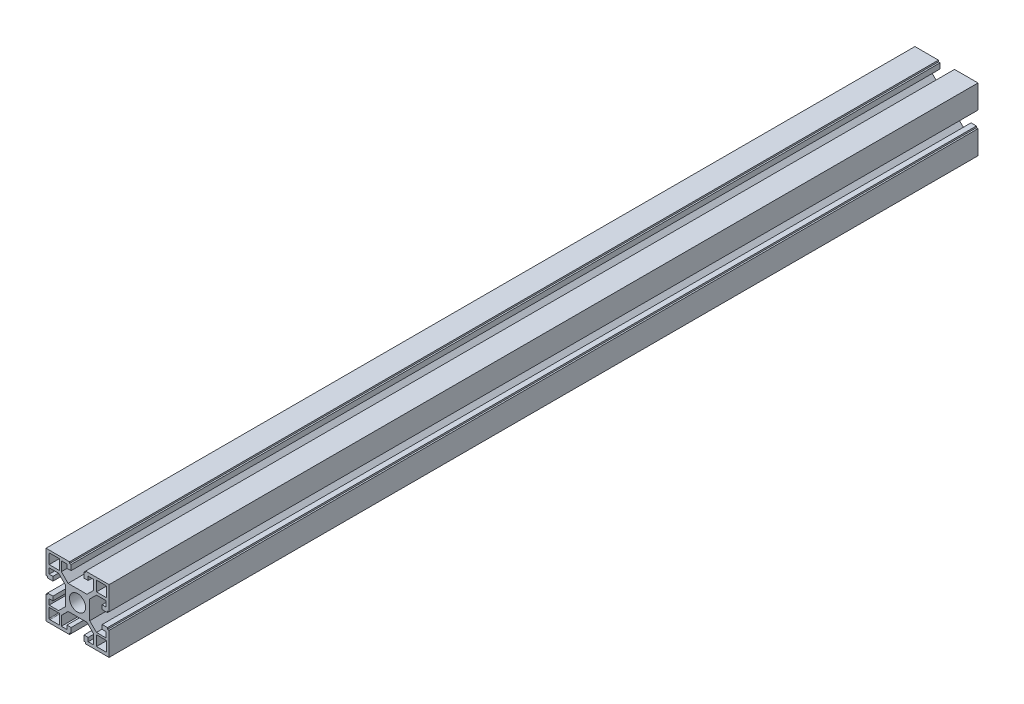
SolidWorks part; units mm, degrees
ref_plane "前视基准面" through (0, 0, 0) normal (0, 0, 1) x (1, 0, 0)
ref_plane "上视基准面" through (0, 0, 0) normal (0, 1, 0) x (1, 0, 0)
ref_plane "右视基准面" through (0, 0, 0) normal (1, 0, 0) x (0, 0, -1)
sketch "草图1" plane through (0, 0, 0) normal (0, 0, 1) x (1, 0, 0)
  line L0 (0, 20) -> (0, 0) construction
  line L1 (-20, 20) -> (20, 20)
  line L2 (-20, 20) -> (-20, -20)
  line L3 (-20, -20) -> (20, -20)
  line L4 (20, 20) -> (20, -20)
  line L5 (0, 0) -> (-20, 0) construction
  dimension "D1" = 40
  dimension "D2" = 40
extrude "凸台-拉伸1" add sketch "草图1" along normal blind 551
hole_wizard "Ø6.5 (6.5) 直径孔1" positions "草图3" profile "草图2" hole size "Ø6.5" standard "Gb" end condition through all
sketch "草图3" plane through (0, 0, 551) normal (0, 0, 1) x (1, 0, 0)
  line L0 (-20, 20) -> (-20, -20) construction
  line L1 (-20, -20) -> (20, -20) construction
  point P0 (0, 0)
  dimension "D1" = 20
  dimension "D2" = 20
sketch "草图2" plane through (0, 0, 551) normal (1, 0, 0) x (0, -1, 0)
  line L0 (0, 0) -> (0, 551)
  line L1 (0, 551) -> (3.25, 551)
  line L2 (3.25, 551) -> (3.25, 0)
  line L5 (3.25, 0) -> (0, 0)
  line L11 (0, -6.35) -> (0, 107.95) construction
  dimension "通孔孔直径" = 6.5
  dimension "通孔孔深度" = 551
sketch "草图4" plane through (0, 0, 551) normal (0, 0, 1) x (1, 0, 0)
  line L0 (0, 0) -> (0, -44.3335) construction
  line L1 (0, 0) -> (0, -7.7) construction
  line L2 (6, -7.7) -> (10.25, -12)
  line L3 (10.25, -12) -> (10.25, -18)
  line L4 (10.25, -18) -> (6.75, -18)
  line L5 (6.75, -18) -> (6.75, -15.6)
  line L6 (6.75, -15.6) -> (4.1, -15.6)
  line L7 (4.1, -15.6) -> (4.1, -19)
  line L8 (4.1, -19) -> (5.1, -19)
  line L9 (5.1, -19) -> (5.1, -23.7257)
  line L10 (5.1, -23.7257) -> (-5.1, -23.7257)
  line L11 (-5.1, -23.7257) -> (-5.1, -19)
  line L12 (-5.1, -19) -> (-4.1, -19)
  line L13 (-4.1, -19) -> (-4.1, -15.6)
  line L14 (-4.1, -15.6) -> (-6.75, -15.6)
  line L15 (-6.75, -15.6) -> (-6.75, -18)
  line L16 (-6.75, -18) -> (-10.25, -18)
  line L17 (-10.25, -18) -> (-10.25, -12)
  line L18 (-10.25, -12) -> (-6, -7.7)
  line L19 (-6, -7.7) -> (6, -7.7)
  line L20 (-20, -20) -> (20, -20) construction
  dimension "D1" = 10.2
  dimension "D2" = 8.2
  dimension "D3" = 20.5
  dimension "D4" = 12.3
  dimension "D5" = 2
  dimension "D6" = 4.4
  dimension "D7" = 1
  dimension "D8" = 13.5
  dimension "D9" = 12
  dimension "D10" = 8
extrude "切除-拉伸1" cut sketch "草图4" against normal through all
pattern_circular "阵列(圆周)1" count 4 every 90 about axis through (0, 0, 0) along (0, 0, 1) of "切除-拉伸1"
sketch "草图5" plane through (0, 0, 0) normal (0, 0, -1) x (-1, 0, 0)
  line L0 (20, -5.1) -> (20, -20) construction
  line L1 (11.5, -11.5) -> (18, -11.5)
  line L2 (11.5, -11.5) -> (11.5, -18)
  line L3 (11.5, -18) -> (18, -18)
  line L4 (18, -11.5) -> (18, -18)
  line L5 (20, -20) -> (5.1, -20) construction
  dimension "D1" = 6.5
  dimension "D2" = 6.5
  dimension "D3" = 2
  dimension "D4" = 2
extrude "切除-拉伸2" cut sketch "草图5" against normal through all
pattern_linear "阵列(线性)1" count 2 spacing 30 along (1, 0, 0) count 2 spacing 30 along (0, 1, 0) of "切除-拉伸2"
fillet "圆角1" [suppressed] radius 2.5
fillet "圆角2" radius 0.5 4 edges at (-18, -18, 275.5) (18.5, -18, 275.5) (18.5, 18.5, 275.5) (-18, 18.5, 275.5)
hole_wizard "M12 螺纹孔1" positions "草图7" profile "草图6" tap size "M12" standard "Iso"
sketch "草图7" plane through (0, 0, 551) normal (0, 0, 1) x (1, 0, 0)
  point P0 (0, 0)
sketch "草图6" plane through (0, 0, 551) normal (1, 0, 0) x (0, -1, 0)
  line L0 (0, 0) -> (0, 32.3144)
  line L1 (0, 32.3144) -> (5.1, 29.25)
  line L2 (5.1, 29.25) -> (5.1, 0)
  line L5 (5.1, 0) -> (0, 0)
  line L10 (0, 32.3144) -> (-5.1, 29.25) construction
  line L11 (0, -6.35) -> (0, 107.95) construction
  dimension "螺纹孔钻头直径" = 10.2
  dimension "螺纹孔钻头深度" = 29.25
  dimension "导头角度" = 118
cosmetic thread "孔螺蚊线1" parameters "D1"=24, "D2"=12
hole_wizard "M8 螺纹孔2" positions "草图9" profile "草图8" tap size "M8" standard "Gb"
sketch "草图9" plane through (0, 0, 0) normal (0, 0, -1) x (-1, 0, 0)
  point P0 (0, 0)
sketch "草图8" plane through (0, 0, 0) normal (1, 0, 0) x (0, 1, 0)
  line L0 (0, 0) -> (0, 21.7929)
  line L1 (0, 21.7929) -> (3.4, 19.75)
  line L2 (3.4, 19.75) -> (3.4, 0)
  line L5 (3.4, 0) -> (0, 0)
  line L10 (0, 21.7929) -> (-3.4, 19.75) construction
  line L11 (0, -6.35) -> (0, 107.95) construction
  dimension "螺纹孔钻头直径" = 6.8
  dimension "螺纹孔钻头深度" = 19.75
  dimension "导头角度" = 118
cosmetic thread "孔螺蚊线2" parameters "D1"=16, "D2"=8
